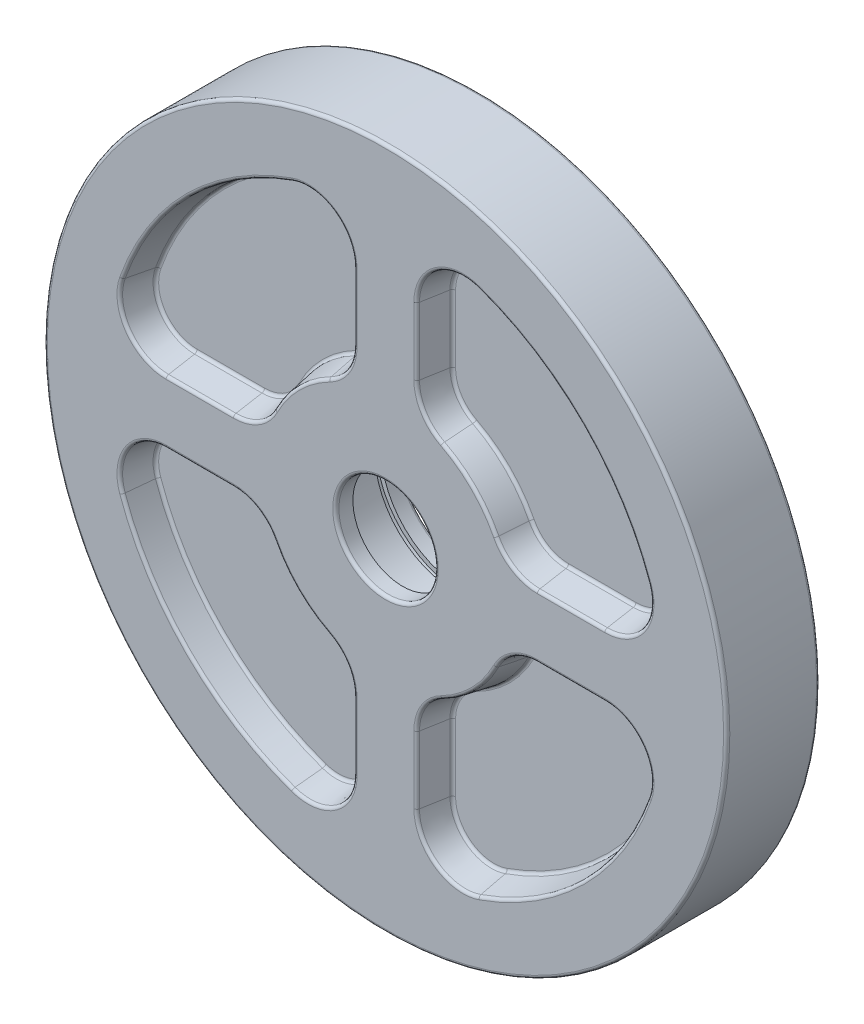
from build123d import *

# Parameters (mm, degrees)
SKETCH1_R                = 110
BOSS_EXTRUDE1_DEPTH      = 15
SKETCH2_R                = 16
CUT_EXTRUDE1_DEPTH       = 5.5
SKETCH3_R                = 22.5
CUT_EXTRUDE2_DEPTH       = 2
SKETCH4_R                = 26
CUT_EXTRUDE3_DEPTH       = 15
SKETCH5_R                = 27.5
CUT_EXTRUDE4_DEPTH       = 2
SKETCH6_R                = 26
CUT_EXTRUDE5_DEPTH       = 158.480951229
CUT_EXTRUDE6_DEPTH       = 10
CUT_EXTRUDE6_DRAFT       = -10
CIRPATTERN1_COPY_1_DEPTH = 10
CIRPATTERN1_COPY_1_DRAFT = -10
CIRPATTERN1_COPY_2_DEPTH = 10
CIRPATTERN1_COPY_2_DRAFT = -10
CIRPATTERN1_COPY_3_DEPTH = 10
CIRPATTERN1_COPY_3_DRAFT = -10
MIRROR1_COPY_1_DEPTH     = 10
MIRROR1_COPY_1_DRAFT     = -10
MIRROR1_COPY_2_DEPTH     = 10
MIRROR1_COPY_2_DRAFT     = -10
MIRROR1_COPY_3_DEPTH     = 10
MIRROR1_COPY_3_DRAFT     = -10
MIRROR1_COPY_4_DEPTH     = 10
MIRROR1_COPY_4_DRAFT     = -10
FILLET1_R                = 1
FILLET2_R                = 1
SKETCH8_R                = 1.5
CUT_EXTRUDE7_DEPTH       = 10


with BuildPart() as part:
    # Sketch1 → Boss-Extrude1 (new, symmetric)
    with BuildSketch(Plane.XY):
        Circle(SKETCH1_R)
    extrude(amount=BOSS_EXTRUDE1_DEPTH, both=True)

    # Sketch2 → Cut-Extrude1 (cut)
    with BuildSketch(Plane.XY.offset(15)):
        Circle(SKETCH2_R)
    extrude(amount=-CUT_EXTRUDE1_DEPTH, mode=Mode.SUBTRACT)

    # Sketch3 → Cut-Extrude2 (cut)
    with BuildSketch(Plane.XY.offset(9.5)):
        Circle(SKETCH3_R)
    extrude(amount=-CUT_EXTRUDE2_DEPTH, mode=Mode.SUBTRACT)

    # Sketch4 → Cut-Extrude3 (cut)
    with BuildSketch(Plane.XY.offset(7.5)):
        Circle(SKETCH4_R)
    extrude(amount=-CUT_EXTRUDE3_DEPTH, mode=Mode.SUBTRACT)

    # Sketch5 → Cut-Extrude4 (cut)
    with BuildSketch(Plane.XY.offset(-7.5)):
        Circle(SKETCH5_R)
    extrude(amount=-CUT_EXTRUDE4_DEPTH, mode=Mode.SUBTRACT)

    # Sketch6 → Cut-Extrude5 (cut, through all)
    with BuildSketch(Plane.XY.offset(-9.5)):
        Circle(SKETCH6_R)
    extrude(amount=-CUT_EXTRUDE5_DEPTH, mode=Mode.SUBTRACT)


with BuildPart() as cut_extrude6_tool:
    # Sketch7 → Cut-Extrude6 (with draft: the straight prism first)
    with BuildSketch(Plane(origin=(0, 0, -15), x_dir=(-1, 0, 0), z_dir=(0, 0, -1))):
        with BuildLine():
            ThreePointArc((-10, 70.710678119), (-16.339745962, 82.958126833), (-30, 84.852813742))
            ThreePointArc((-30, 84.852813742), (-63.639610307, 63.639610307), (-84.852813742, 30))
            ThreePointArc((-84.852813742, 30), (-82.958126833, 16.339745962), (-70.710678119, 10))
            Line((-70.710678119, 10), (-48.989794856, 10))
            ThreePointArc((-48.989794856, 10), (-41.156300338, 12.207957019), (-35.628941713, 18.181818182))
            ThreePointArc((-35.628941713, 18.181818182), (-28.284271247, 28.284271247), (-18.181818182, 35.628941713))
            ThreePointArc((-18.181818182, 35.628941713), (-12.207957019, 41.156300338), (-10, 48.989794856))
            Line((-10, 48.989794856), (-10, 70.710678119))
        make_face()
    extrude(amount=-CUT_EXTRUDE6_DEPTH)
    # Cut-Extrude6: the draft: its side faces are tilted about the plane it starts from
    cut_extrude6_sides = [cut_extrude6_tool.faces().sort_by_distance(p)[0] for p in [
        (12.207957019, 41.156300338, -10),
        (10, 59.850236487, -10),
        (16.339745962, 82.958126833, -10),
        (63.639610307, 63.639610307, -10),
        (82.958126833, 16.339745962, -10),
        (59.850236487, 10, -10),
        (41.156300338, 12.207957019, -10),
        (28.284271247, 28.284271247, -10),
    ]]
    draft(cut_extrude6_sides, Plane(origin=(0, 0, -15), x_dir=(-1, 0, 0), z_dir=(0, 0, -1)), CUT_EXTRUDE6_DRAFT)


with BuildPart() as part_1:
    add(part.part)

    # Cut-Extrude6: cut by cut_extrude6_tool
    add(cut_extrude6_tool.part, mode=Mode.SUBTRACT)


with BuildPart() as cirpattern1_copy_1_tool:
    # CirPattern1 copy 1 sketch → CirPattern1 copy 1 (with draft: the straight prism first)
    with BuildSketch(Plane(origin=(0, 0, -15), x_dir=(0, -1, 0), z_dir=(0, 0, -1))):
        with BuildLine():
            ThreePointArc((-10, 70.710678119), (-16.339745962, 82.958126833), (-30, 84.852813742))
            ThreePointArc((-30, 84.852813742), (-63.639610307, 63.639610307), (-84.852813742, 30))
            ThreePointArc((-84.852813742, 30), (-82.958126833, 16.339745962), (-70.710678119, 10))
            Line((-70.710678119, 10), (-48.989794856, 10))
            ThreePointArc((-48.989794856, 10), (-41.156300338, 12.207957019), (-35.628941713, 18.181818182))
            ThreePointArc((-35.628941713, 18.181818182), (-28.284271247, 28.284271247), (-18.181818182, 35.628941713))
            ThreePointArc((-18.181818182, 35.628941713), (-12.207957019, 41.156300338), (-10, 48.989794856))
            Line((-10, 48.989794856), (-10, 70.710678119))
        make_face()
    extrude(amount=-CIRPATTERN1_COPY_1_DEPTH)
    # CirPattern1 copy 1: the draft: its side faces are tilted about the plane it starts from
    cirpattern1_copy_1_sides = [cirpattern1_copy_1_tool.faces().sort_by_distance(p)[0] for p in [
        (-41.156300338, 12.207957019, -10),
        (-59.850236487, 10, -10),
        (-82.958126833, 16.339745962, -10),
        (-63.639610307, 63.639610307, -10),
        (-16.339745962, 82.958126833, -10),
        (-10, 59.850236487, -10),
        (-12.207957019, 41.156300338, -10),
        (-28.284271247, 28.284271247, -10),
    ]]
    draft(cirpattern1_copy_1_sides, Plane(origin=(0, 0, -15), x_dir=(0, -1, 0), z_dir=(0, 0, -1)), CIRPATTERN1_COPY_1_DRAFT)


with BuildPart() as part_2:
    add(part_1.part)

    # CirPattern1 copy 1: cut by cirpattern1_copy_1_tool
    add(cirpattern1_copy_1_tool.part, mode=Mode.SUBTRACT)


with BuildPart() as cirpattern1_copy_2_tool:
    # CirPattern1 copy 2 sketch → CirPattern1 copy 2 (with draft: the straight prism first)
    with BuildSketch(Plane(origin=(0, 0, -15), x_dir=(1, 0, 0), z_dir=(0, 0, -1))):
        with BuildLine():
            ThreePointArc((-10, 70.710678119), (-16.339745962, 82.958126833), (-30, 84.852813742))
            ThreePointArc((-30, 84.852813742), (-63.639610307, 63.639610307), (-84.852813742, 30))
            ThreePointArc((-84.852813742, 30), (-82.958126833, 16.339745962), (-70.710678119, 10))
            Line((-70.710678119, 10), (-48.989794856, 10))
            ThreePointArc((-48.989794856, 10), (-41.156300338, 12.207957019), (-35.628941713, 18.181818182))
            ThreePointArc((-35.628941713, 18.181818182), (-28.284271247, 28.284271247), (-18.181818182, 35.628941713))
            ThreePointArc((-18.181818182, 35.628941713), (-12.207957019, 41.156300338), (-10, 48.989794856))
            Line((-10, 48.989794856), (-10, 70.710678119))
        make_face()
    extrude(amount=-CIRPATTERN1_COPY_2_DEPTH)
    # CirPattern1 copy 2: the draft: its side faces are tilted about the plane it starts from
    cirpattern1_copy_2_sides = [cirpattern1_copy_2_tool.faces().sort_by_distance(p)[0] for p in [
        (-12.207957019, -41.156300338, -10),
        (-10, -59.850236487, -10),
        (-16.339745962, -82.958126833, -10),
        (-63.639610307, -63.639610307, -10),
        (-82.958126833, -16.339745962, -10),
        (-59.850236487, -10, -10),
        (-41.156300338, -12.207957019, -10),
        (-28.284271247, -28.284271247, -10),
    ]]
    draft(cirpattern1_copy_2_sides, Plane(origin=(0, 0, -15), x_dir=(1, 0, 0), z_dir=(0, 0, -1)), CIRPATTERN1_COPY_2_DRAFT)


with BuildPart() as part_3:
    add(part_2.part)

    # CirPattern1 copy 2: cut by cirpattern1_copy_2_tool
    add(cirpattern1_copy_2_tool.part, mode=Mode.SUBTRACT)


with BuildPart() as cirpattern1_copy_3_tool:
    # CirPattern1 copy 3 sketch → CirPattern1 copy 3 (with draft: the straight prism first)
    with BuildSketch(Plane.YX.offset(15)):
        with BuildLine():
            ThreePointArc((-10, 70.710678119), (-16.339745962, 82.958126833), (-30, 84.852813742))
            ThreePointArc((-30, 84.852813742), (-63.639610307, 63.639610307), (-84.852813742, 30))
            ThreePointArc((-84.852813742, 30), (-82.958126833, 16.339745962), (-70.710678119, 10))
            Line((-70.710678119, 10), (-48.989794856, 10))
            ThreePointArc((-48.989794856, 10), (-41.156300338, 12.207957019), (-35.628941713, 18.181818182))
            ThreePointArc((-35.628941713, 18.181818182), (-28.284271247, 28.284271247), (-18.181818182, 35.628941713))
            ThreePointArc((-18.181818182, 35.628941713), (-12.207957019, 41.156300338), (-10, 48.989794856))
            Line((-10, 48.989794856), (-10, 70.710678119))
        make_face()
    extrude(amount=-CIRPATTERN1_COPY_3_DEPTH)
    # CirPattern1 copy 3: the draft: its side faces are tilted about the plane it starts from
    cirpattern1_copy_3_sides = [cirpattern1_copy_3_tool.faces().sort_by_distance(p)[0] for p in [
        (41.156300338, -12.207957019, -10),
        (59.850236487, -10, -10),
        (82.958126833, -16.339745962, -10),
        (63.639610307, -63.639610307, -10),
        (16.339745962, -82.958126833, -10),
        (10, -59.850236487, -10),
        (12.207957019, -41.156300338, -10),
        (28.284271247, -28.284271247, -10),
    ]]
    draft(cirpattern1_copy_3_sides, Plane.YX.offset(15), CIRPATTERN1_COPY_3_DRAFT)


with BuildPart() as part_4:
    add(part_3.part)

    # CirPattern1 copy 3: cut by cirpattern1_copy_3_tool
    add(cirpattern1_copy_3_tool.part, mode=Mode.SUBTRACT)


with BuildPart() as mirror1_copy_1_tool:
    # Mirror1 copy 1 sketch → Mirror1 copy 1 (with draft: the straight prism first)
    with BuildSketch(Plane(origin=(0, 0, 15), x_dir=(-1, 0, 0), z_dir=(0, 0, 1))):
        with BuildLine():
            ThreePointArc((-10, -70.710678119), (-16.339745962, -82.958126833), (-30, -84.852813742))
            ThreePointArc((-30, -84.852813742), (-63.639610307, -63.639610307), (-84.852813742, -30))
            ThreePointArc((-84.852813742, -30), (-82.958126833, -16.339745962), (-70.710678119, -10))
            Line((-70.710678119, -10), (-48.989794856, -10))
            ThreePointArc((-48.989794856, -10), (-41.156300338, -12.207957019), (-35.628941713, -18.181818182))
            ThreePointArc((-35.628941713, -18.181818182), (-28.284271247, -28.284271247), (-18.181818182, -35.628941713))
            ThreePointArc((-18.181818182, -35.628941713), (-12.207957019, -41.156300338), (-10, -48.989794856))
            Line((-10, -48.989794856), (-10, -70.710678119))
        make_face()
    extrude(amount=-MIRROR1_COPY_1_DEPTH)
    # Mirror1 copy 1: the draft: its side faces are tilted about the plane it starts from
    mirror1_copy_1_sides = [mirror1_copy_1_tool.faces().sort_by_distance(p)[0] for p in [
        (12.207957019, 41.156300338, 10),
        (10, 59.850236487, 10),
        (16.339745962, 82.958126833, 10),
        (63.639610307, 63.639610307, 10),
        (82.958126833, 16.339745962, 10),
        (59.850236487, 10, 10),
        (41.156300338, 12.207957019, 10),
        (28.284271247, 28.284271247, 10),
    ]]
    draft(mirror1_copy_1_sides, Plane(origin=(0, 0, 15), x_dir=(-1, 0, 0), z_dir=(0, 0, 1)), MIRROR1_COPY_1_DRAFT)


with BuildPart() as part_5:
    add(part_4.part)

    # Mirror1 copy 1: cut by mirror1_copy_1_tool
    add(mirror1_copy_1_tool.part, mode=Mode.SUBTRACT)


with BuildPart() as mirror1_copy_2_tool:
    # Mirror1 copy 2 sketch → Mirror1 copy 2 (with draft: the straight prism first)
    with BuildSketch(Plane(origin=(0, 0, 15), x_dir=(0, -1, 0), z_dir=(0, 0, 1))):
        with BuildLine():
            ThreePointArc((-10, -70.710678119), (-16.339745962, -82.958126833), (-30, -84.852813742))
            ThreePointArc((-30, -84.852813742), (-63.639610307, -63.639610307), (-84.852813742, -30))
            ThreePointArc((-84.852813742, -30), (-82.958126833, -16.339745962), (-70.710678119, -10))
            Line((-70.710678119, -10), (-48.989794856, -10))
            ThreePointArc((-48.989794856, -10), (-41.156300338, -12.207957019), (-35.628941713, -18.181818182))
            ThreePointArc((-35.628941713, -18.181818182), (-28.284271247, -28.284271247), (-18.181818182, -35.628941713))
            ThreePointArc((-18.181818182, -35.628941713), (-12.207957019, -41.156300338), (-10, -48.989794856))
            Line((-10, -48.989794856), (-10, -70.710678119))
        make_face()
    extrude(amount=-MIRROR1_COPY_2_DEPTH)
    # Mirror1 copy 2: the draft: its side faces are tilted about the plane it starts from
    mirror1_copy_2_sides = [mirror1_copy_2_tool.faces().sort_by_distance(p)[0] for p in [
        (-41.156300338, 12.207957019, 10),
        (-59.850236487, 10, 10),
        (-82.958126833, 16.339745962, 10),
        (-63.639610307, 63.639610307, 10),
        (-16.339745962, 82.958126833, 10),
        (-10, 59.850236487, 10),
        (-12.207957019, 41.156300338, 10),
        (-28.284271247, 28.284271247, 10),
    ]]
    draft(mirror1_copy_2_sides, Plane(origin=(0, 0, 15), x_dir=(0, -1, 0), z_dir=(0, 0, 1)), MIRROR1_COPY_2_DRAFT)


with BuildPart() as part_6:
    add(part_5.part)

    # Mirror1 copy 2: cut by mirror1_copy_2_tool
    add(mirror1_copy_2_tool.part, mode=Mode.SUBTRACT)


with BuildPart() as mirror1_copy_3_tool:
    # Mirror1 copy 3 sketch → Mirror1 copy 3 (with draft: the straight prism first)
    with BuildSketch(Plane.XY.offset(15)):
        with BuildLine():
            ThreePointArc((-10, -70.710678119), (-16.339745962, -82.958126833), (-30, -84.852813742))
            ThreePointArc((-30, -84.852813742), (-63.639610307, -63.639610307), (-84.852813742, -30))
            ThreePointArc((-84.852813742, -30), (-82.958126833, -16.339745962), (-70.710678119, -10))
            Line((-70.710678119, -10), (-48.989794856, -10))
            ThreePointArc((-48.989794856, -10), (-41.156300338, -12.207957019), (-35.628941713, -18.181818182))
            ThreePointArc((-35.628941713, -18.181818182), (-28.284271247, -28.284271247), (-18.181818182, -35.628941713))
            ThreePointArc((-18.181818182, -35.628941713), (-12.207957019, -41.156300338), (-10, -48.989794856))
            Line((-10, -48.989794856), (-10, -70.710678119))
        make_face()
    extrude(amount=-MIRROR1_COPY_3_DEPTH)
    # Mirror1 copy 3: the draft: its side faces are tilted about the plane it starts from
    mirror1_copy_3_sides = [mirror1_copy_3_tool.faces().sort_by_distance(p)[0] for p in [
        (-12.207957019, -41.156300338, 10),
        (-10, -59.850236487, 10),
        (-16.339745962, -82.958126833, 10),
        (-63.639610307, -63.639610307, 10),
        (-82.958126833, -16.339745962, 10),
        (-59.850236487, -10, 10),
        (-41.156300338, -12.207957019, 10),
        (-28.284271247, -28.284271247, 10),
    ]]
    draft(mirror1_copy_3_sides, Plane.XY.offset(15), MIRROR1_COPY_3_DRAFT)


with BuildPart() as part_7:
    add(part_6.part)

    # Mirror1 copy 3: cut by mirror1_copy_3_tool
    add(mirror1_copy_3_tool.part, mode=Mode.SUBTRACT)


with BuildPart() as mirror1_copy_4_tool:
    # Mirror1 copy 4 sketch → Mirror1 copy 4 (with draft: the straight prism first)
    with BuildSketch(Plane(origin=(0, 0, 15), x_dir=(0, 1, 0), z_dir=(0, 0, 1))):
        with BuildLine():
            ThreePointArc((-10, -70.710678119), (-16.339745962, -82.958126833), (-30, -84.852813742))
            ThreePointArc((-30, -84.852813742), (-63.639610307, -63.639610307), (-84.852813742, -30))
            ThreePointArc((-84.852813742, -30), (-82.958126833, -16.339745962), (-70.710678119, -10))
            Line((-70.710678119, -10), (-48.989794856, -10))
            ThreePointArc((-48.989794856, -10), (-41.156300338, -12.207957019), (-35.628941713, -18.181818182))
            ThreePointArc((-35.628941713, -18.181818182), (-28.284271247, -28.284271247), (-18.181818182, -35.628941713))
            ThreePointArc((-18.181818182, -35.628941713), (-12.207957019, -41.156300338), (-10, -48.989794856))
            Line((-10, -48.989794856), (-10, -70.710678119))
        make_face()
    extrude(amount=-MIRROR1_COPY_4_DEPTH)
    # Mirror1 copy 4: the draft: its side faces are tilted about the plane it starts from
    mirror1_copy_4_sides = [mirror1_copy_4_tool.faces().sort_by_distance(p)[0] for p in [
        (41.156300338, -12.207957019, 10),
        (59.850236487, -10, 10),
        (82.958126833, -16.339745962, 10),
        (63.639610307, -63.639610307, 10),
        (16.339745962, -82.958126833, 10),
        (10, -59.850236487, 10),
        (12.207957019, -41.156300338, 10),
        (28.284271247, -28.284271247, 10),
    ]]
    draft(mirror1_copy_4_sides, Plane(origin=(0, 0, 15), x_dir=(0, 1, 0), z_dir=(0, 0, 1)), MIRROR1_COPY_4_DRAFT)


with BuildPart() as part_8:
    add(part_7.part)

    # Mirror1 copy 4: cut by mirror1_copy_4_tool
    add(mirror1_copy_4_tool.part, mode=Mode.SUBTRACT)

    # Fillet1
    fillet1_edges = [part_8.edges().sort_by_distance(p)[0] for p in [
        (-110, 0, -15),
        (-26, 0, -15),
        (42.077137962, 13.711678563, -5),
        (59.850236487, 11.763269807, -5),
        (81.518423064, 17.35777026, -5),
        (62.392790269, 62.392790269, -5),
        (17.35777026, 81.518423064, -5),
        (11.763269807, 59.850236487, -5),
        (13.711678563, 42.077137962, -5),
        (29.531091285, 29.531091285, -5),
        (41.156300338, 12.207957019, -15),
        (28.284271247, 28.284271247, -15),
        (12.207957019, 41.156300338, -15),
        (10, 59.850236487, -15),
        (16.339745962, 82.958126833, -15),
        (63.639610307, 63.639610307, -15),
        (82.958126833, 16.339745962, -15),
        (59.850236487, 10, -15),
        (13.711678563, -42.077137962, -5),
        (11.763269807, -59.850236487, -5),
        (17.35777026, -81.518423064, -5),
        (62.392790269, -62.392790269, -5),
        (81.518423064, -17.35777026, -5),
        (59.850236487, -11.763269807, -5),
        (42.077137962, -13.711678563, -5),
        (29.531091285, -29.531091285, -5),
        (12.207957019, -41.156300338, -15),
        (28.284271247, -28.284271247, -15),
        (41.156300338, -12.207957019, -15),
        (59.850236487, -10, -15),
        (82.958126833, -16.339745962, -15),
        (63.639610307, -63.639610307, -15),
        (16.339745962, -82.958126833, -15),
        (10, -59.850236487, -15),
        (-42.077137962, -13.711678563, -5),
        (-59.850236487, -11.763269807, -5),
        (-81.518423064, -17.35777026, -5),
        (-62.392790269, -62.392790269, -5),
        (-17.35777026, -81.518423064, -5),
        (-11.763269807, -59.850236487, -5),
        (-13.711678563, -42.077137962, -5),
        (-29.531091285, -29.531091285, -5),
        (-41.156300338, -12.207957019, -15),
        (-28.284271247, -28.284271247, -15),
        (-12.207957019, -41.156300338, -15),
        (-10, -59.850236487, -15),
        (-16.339745962, -82.958126833, -15),
        (-63.639610307, -63.639610307, -15),
        (-82.958126833, -16.339745962, -15),
        (-59.850236487, -10, -15),
        (-13.711678563, 42.077137962, -5),
        (-11.763269807, 59.850236487, -5),
        (-17.35777026, 81.518423064, -5),
        (-62.392790269, 62.392790269, -5),
        (-81.518423064, 17.35777026, -5),
        (-59.850236487, 11.763269807, -5),
        (-42.077137962, 13.711678563, -5),
        (-29.531091285, 29.531091285, -5),
        (-12.207957019, 41.156300338, -15),
        (-28.284271247, 28.284271247, -15),
        (-41.156300338, 12.207957019, -15),
        (-59.850236487, 10, -15),
        (-82.958126833, 16.339745962, -15),
        (-63.639610307, 63.639610307, -15),
        (-16.339745962, 82.958126833, -15),
        (-10, 59.850236487, -15),
    ]]
    fillet(fillet1_edges, radius=FILLET1_R)

    # Fillet2
    fillet2_edges = [part_8.edges().sort_by_distance(p)[0] for p in [
        (41.156300338, 12.207957019, 15),
        (28.284271247, 28.284271247, 15),
        (12.207957019, 41.156300338, 15),
        (10, 59.850236487, 15),
        (16.339745962, 82.958126833, 15),
        (63.639610307, 63.639610307, 15),
        (82.958126833, 16.339745962, 15),
        (59.850236487, 10, 15),
        (42.077137962, 13.711678563, 5),
        (29.531091285, 29.531091285, 5),
        (13.711678563, 42.077137962, 5),
        (11.763269807, 59.850236487, 5),
        (17.35777026, 81.518423064, 5),
        (62.392790269, 62.392790269, 5),
        (81.518423064, 17.35777026, 5),
        (59.850236487, 11.763269807, 5),
        (12.207957019, -41.156300338, 15),
        (28.284271247, -28.284271247, 15),
        (41.156300338, -12.207957019, 15),
        (59.850236487, -10, 15),
        (82.958126833, -16.339745962, 15),
        (63.639610307, -63.639610307, 15),
        (16.339745962, -82.958126833, 15),
        (10, -59.850236487, 15),
        (13.711678563, -42.077137962, 5),
        (29.531091285, -29.531091285, 5),
        (42.077137962, -13.711678563, 5),
        (59.850236487, -11.763269807, 5),
        (81.518423064, -17.35777026, 5),
        (62.392790269, -62.392790269, 5),
        (17.35777026, -81.518423064, 5),
        (11.763269807, -59.850236487, 5),
        (-41.156300338, -12.207957019, 15),
        (-28.284271247, -28.284271247, 15),
        (-12.207957019, -41.156300338, 15),
        (-10, -59.850236487, 15),
        (-16.339745962, -82.958126833, 15),
        (-63.639610307, -63.639610307, 15),
        (-82.958126833, -16.339745962, 15),
        (-59.850236487, -10, 15),
        (-42.077137962, -13.711678563, 5),
        (-29.531091285, -29.531091285, 5),
        (-13.711678563, -42.077137962, 5),
        (-11.763269807, -59.850236487, 5),
        (-17.35777026, -81.518423064, 5),
        (-62.392790269, -62.392790269, 5),
        (-81.518423064, -17.35777026, 5),
        (-59.850236487, -11.763269807, 5),
        (-12.207957019, 41.156300338, 15),
        (-28.284271247, 28.284271247, 15),
        (-41.156300338, 12.207957019, 15),
        (-59.850236487, 10, 15),
        (-82.958126833, 16.339745962, 15),
        (-63.639610307, 63.639610307, 15),
        (-16.339745962, 82.958126833, 15),
        (-10, 59.850236487, 15),
        (-13.711678563, 42.077137962, 5),
        (-29.531091285, 29.531091285, 5),
        (-42.077137962, 13.711678563, 5),
        (-59.850236487, 11.763269807, 5),
        (-81.518423064, 17.35777026, 5),
        (-62.392790269, 62.392790269, 5),
        (-17.35777026, 81.518423064, 5),
        (-11.763269807, 59.850236487, 5),
        (-110, 0, 15),
        (-16, 0, 15),
    ]]
    fillet(fillet2_edges, radius=FILLET2_R)

    # Sketch8 → Cut-Extrude7 (cut)
    with BuildSketch(Plane(origin=(0, 0, -15), x_dir=(-1, 0, 0), z_dir=(0, 0, -1))):
        with Locations((0, 32.5)):
            Circle(SKETCH8_R)
        with Locations((28.145825623, -16.25)):
            Circle(SKETCH8_R)
        with Locations((-28.145825623, -16.25)):
            Circle(SKETCH8_R)
    extrude(amount=-CUT_EXTRUDE7_DEPTH, mode=Mode.SUBTRACT)


solid = part_8.part
